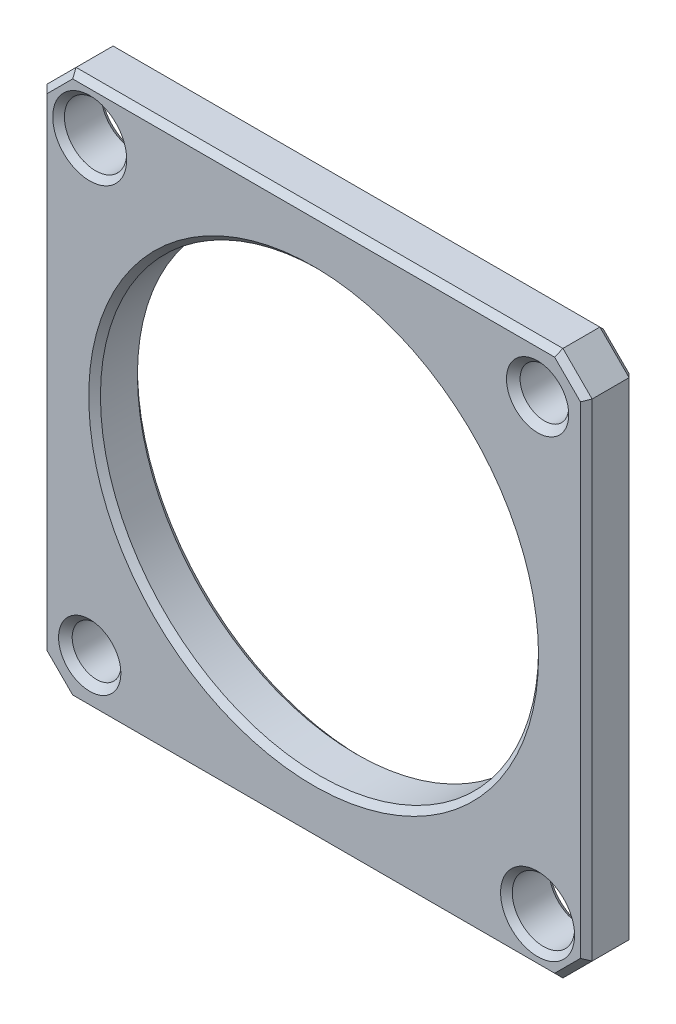
SolidWorks part; units mm, degrees
material "45"
ref_plane "Front Plane" through (0, 0, 0) normal (0, 0, 1) x (1, 0, 0)
ref_plane "Top Plane" through (0, 0, 0) normal (0, 1, 0) x (1, 0, 0)
ref_plane "Right Plane" through (0, 0, 0) normal (1, 0, 0) x (0, 0, -1)
sketch "Sketch1" plane through (0, 0, 0) normal (0, 0, 1) x (1, 0, 0)
  line L0 (-14, -12.5) -> (-12.5, -14)
  line L1 (-12.5, 14) -> (12.5, 14)
  line L2 (-14, 12.5) -> (-14, -12.5)
  line L3 (-12.5, -14) -> (12.5, -14)
  line L4 (14, 12.5) -> (14, -12.5)
  line L5 (-14, 14) -> (14, -14) construction
  line L6 (-14, -14) -> (14, 14) construction
  line L7 (12.5, -14) -> (14, -12.5)
  line L8 (12.5, 14) -> (14, 12.5)
  line L9 (-14, 12.5) -> (-12.5, 14)
  circle A0 centre (0, 0) radius 11.25
  point P0 (0, 0)
  dimension "D3" = 22.5
  dimension "D1" = 28
  dimension "D2" = 28
extrude "Boss-Extrude1" add sketch "Sketch1" along normal blind 2.5
sketch "Sketch2" plane through (0, 0, 2.5) normal (0, 0, 1) x (1, 0, 0)
  line L0 (-11.5, 11.5) -> (0, 0) construction
  line L1 (0, 0) -> (11.5, -11.5) construction
  line L2 (12.5, 14) -> (-12.5, 14) construction
  circle A0 centre (-11.5, 11.5) radius 1.6
  circle A1 centre (11.5, -11.5) radius 1.6
  dimension "D3" = 3.2
  dimension "D1" = 45
  dimension "D2" = 11.5
extrude "Cut-Extrude1" cut sketch "Sketch2" against normal blind 2.5
hole_wizard "M3 Tapped Hole1" positions "Sketch3" profile "Sketch4" tap size "M3" standard "GB" end condition through all
sketch "Sketch3" plane through (0, 0, 2.5) normal (0, 0, 1) x (1, 0, 0)
  line L1 (-11.5, 11.5) -> (11.5, 11.5)
  line L2 (-11.5, -11.5) -> (-11.5, 11.5)
  point P0 (-11.5, -11.5)
  point P2 (11.5, 11.5)
  dimension "D1" = 23
  dimension "D2" = 23
sketch "Sketch4" plane through (-11.5, -11.5, 2.5) normal (1, 0, 0) x (0, -1, 0)
  line L0 (0, 0) -> (0, 2.5)
  line L1 (0, 2.5) -> (1.6, 2.5)
  line L2 (1.25, 2.15) -> (1.25, 0.35)
  line L3 (1.25, 0.35) -> (1.6, 0)
  line L5 (1.6, 0) -> (0, 0)
  line L6 (-1.25, 0.35) -> (-1.6, 0) construction
  line L7 (1.6, 2.5) -> (1.25, 2.15)
  line L8 (-1.6, 2.5) -> (-1.25, 2.15) construction
  line L11 (0, -6.35) -> (0, 107.95) construction
  dimension "通孔螺纹孔钻头直径" = 2.5
  dimension "通孔螺纹孔钻头深度" = 2.5
  dimension "近端锥形沉头孔直径" = 3.2
  dimension "近端锥形沉头孔角度" = 90
  dimension "远端锥形沉头孔直径" = 3.2
  dimension "远端锥形沉头孔角度" = 90
cosmetic thread "Cosmetic Thread1" parameters "D2"=3
cosmetic thread "Cosmetic Thread2" parameters "D2"=3
chamfer "Chamfer1" distance 0.3 angle 45 22 edges at (-13.25, -13.25, 0) (0, -14, 0) (13.25, -13.25, 0) (14, 0, 0) (13.25, 13.25, 0) (0, 14, 0) (-13.25, 13.25, 0) (-14, 0, 0) (11.25, 0, 0) (11.25, 0, 2.5) (0, -14, 2.5) (13.25, -13.25, 2.5) (14, 0, 2.5) (13.25, 13.25, 2.5) (0, 14, 2.5) (-13.25, 13.25, 2.5) (-14, 0, 2.5) (-13.25, -13.25, 2.5) (-9.9, 11.5, 2.5) (-9.9, 11.5, 0) (13.1, -11.5, 2.5) (13.1, -11.5, 0)
